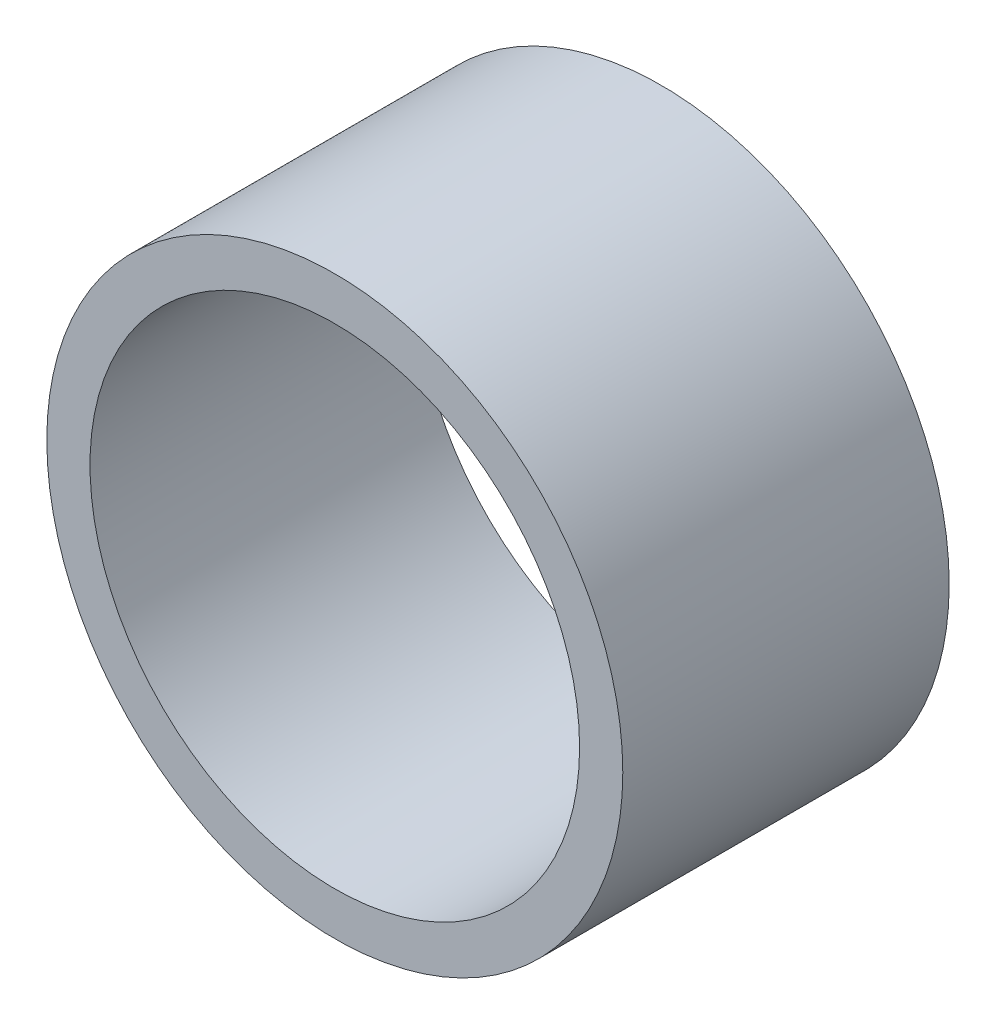
from build123d import *

# Parameters (mm, degrees)
SKETCH_1_R      = 15
SKETCH_1_R_2    = 12.75
EXTRUDE_1_DEPTH = 17


with BuildPart() as part:
    # 草图1 → 凸台-拉伸1 (new body)
    with BuildSketch(Plane.XY):
        Circle(SKETCH_1_R)
        Circle(SKETCH_1_R_2, mode=Mode.SUBTRACT)
    extrude(amount=EXTRUDE_1_DEPTH)


solid = part.part
